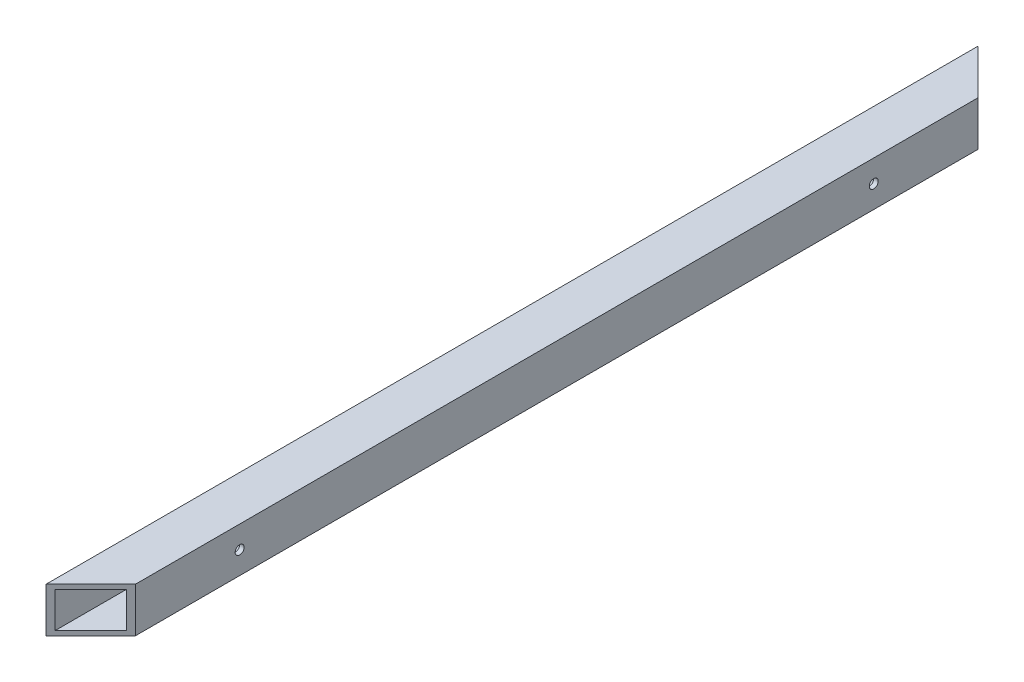
SolidWorks part; units mm, degrees
ref_plane "Front Plane" through (0, 0, 0) normal (0, 0, 1) x (1, 0, 0)
ref_plane "Top Plane" through (0, 0, 0) normal (0, 1, 0) x (1, 0, 0)
ref_plane "Right Plane" through (0, 0, 0) normal (1, 0, 0) x (0, 0, -1)
other "Configuration Table"
sketch "Sketch1" plane through (0, 0, 0) normal (0, 0, 1) x (1, 0, 0)
  line L0 (-42.7737, 46.6218) -> (-12.7737, 46.6218)
  line L1 (-12.7737, 46.6218) -> (-12.7737, 16.6218)
  line L2 (-12.7737, 16.6218) -> (-42.7737, 16.6218)
  line L3 (-42.7737, 16.6218) -> (-42.7737, 46.6218)
extrude "Boss-Extrude1" add sketch "Sketch1" along normal blind 800
sketch "Sketch2" plane through (0, 0, 800) normal (0, 0, 1) x (1, 0, 0)
  line L0 (-39.7737, 43.6218) -> (-15.7737, 43.6218)
  line L1 (-15.7737, 43.6218) -> (-15.7737, 19.6218)
  line L2 (-15.7737, 19.6218) -> (-39.7737, 19.6218)
  line L3 (-39.7737, 19.6218) -> (-39.7737, 43.6218)
  line L4 (-12.7737, 16.6218) -> (-12.7737, 46.6218) construction
  line L5 (-12.7737, 46.6218) -> (-42.7737, 46.6218) construction
  line L6 (-42.7737, 46.6218) -> (-42.7737, 16.6218) construction
  line L7 (-42.7737, 16.6218) -> (-12.7737, 16.6218) construction
  dimension "D1" = 3
  dimension "D2" = 3
  dimension "D3" = 3
  dimension "D4" = 3
extrude "Cut-Extrude1" cut sketch "Sketch2" against normal blind 800
sketch "Sketch3" plane through (0, 16.6218, 0) normal (0, -1, 0) x (-1, 0, 0)
  line L0 (12.7737, -721.6646) -> (42.7737, -751.6646)
  line L1 (12.7737, -800) -> (12.7737, 0) construction
  line L2 (12.7737, -721.6646) -> (-270.0691, -438.8219) construction
  line L3 (42.7737, -800) -> (42.7737, -751.6646)
  line L4 (42.7737, -800) -> (42.7737, 0) construction
  line L5 (42.7737, -800) -> (12.7737, -800)
  line L6 (42.7737, -800) -> (12.7737, -800) construction
  line L7 (12.7737, -800) -> (12.7737, -721.6646)
  line L8 (12.7737, -155.9792) -> (42.7737, -125.9792)
  line L9 (42.7737, -125.9792) -> (42.7737, 0)
  line L10 (42.7737, 0) -> (12.7737, 0)
  line L11 (12.7737, 0) -> (12.7737, -155.9792)
extrude "Cut-Extrude2" cut sketch "Sketch3" against normal through all
sketch "Sketch4" plane through (-48.7737, 0, 0) normal (-1, 0, 0) x (0, 0, 1)
  circle A0 centre (225.9792, 31.6218) radius 3
  circle A1 centre (225.9792, 841.6218) radius 3
  circle A2 centre (651.6646, 841.6218) radius 3
  circle A3 centre (651.6646, 31.6218) radius 3
extrude "Cut-Extrude3" cut sketch "Sketch4" against normal through all
